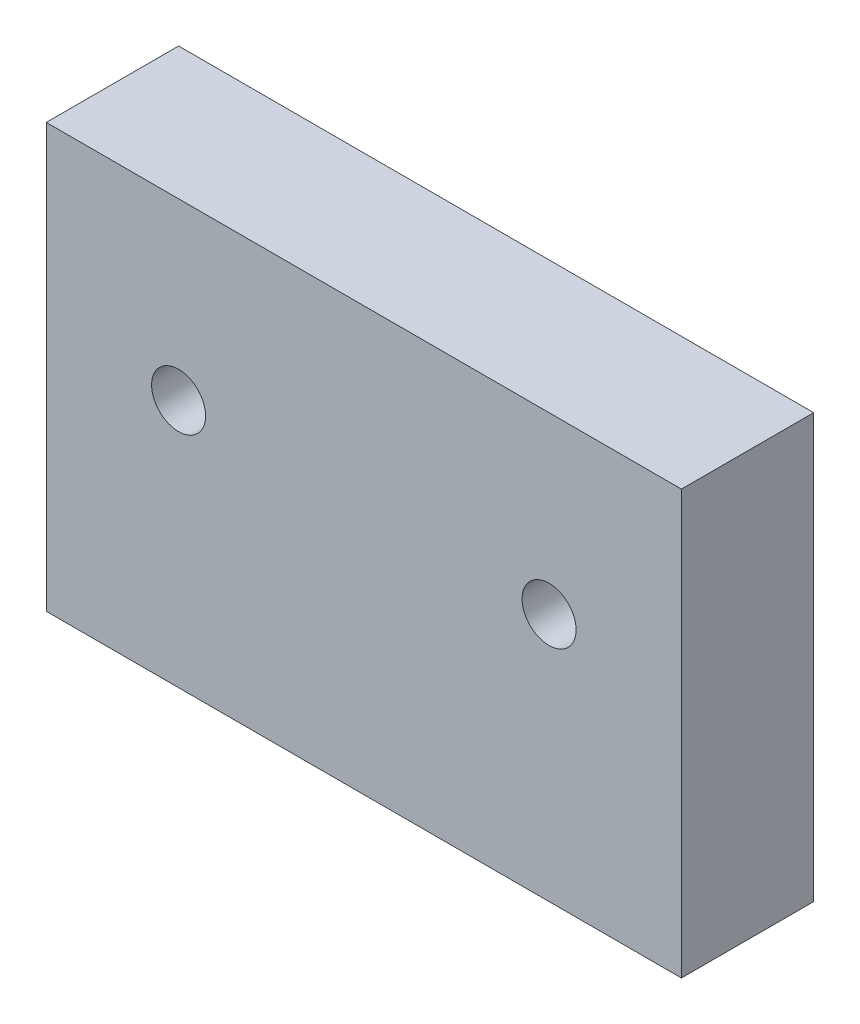
from build123d import *

# Parameters (mm, degrees)
SKETCH1_W              = 120
SKETCH1_H              = 80
BOSS_EXTRUDE1_DEPTH    = 25
M12_TAPPED_HOLE1_D     = 10.2
M12_TAPPED_HOLE1_DEPTH = 29.25
M12_TAPPED_HOLE1_TIP   = 3.064389157


with BuildPart() as part:
    # Sketch1 → Boss-Extrude1 (new body)
    with BuildSketch(Plane.XY):
        Rectangle(SKETCH1_W, SKETCH1_H)
    extrude(amount=BOSS_EXTRUDE1_DEPTH)

    # M12 Tapped Hole1
    with Locations(Plane.XY.offset(25)):
        with Locations((-35, 7), (35, 7)):
            Hole(M12_TAPPED_HOLE1_D / 2, depth=M12_TAPPED_HOLE1_DEPTH)
            with Locations((0, 0, -(M12_TAPPED_HOLE1_DEPTH + M12_TAPPED_HOLE1_TIP / 2))):  # 118° drill point
                Cone(0, M12_TAPPED_HOLE1_D / 2, M12_TAPPED_HOLE1_TIP, mode=Mode.SUBTRACT)


solid = part.part
